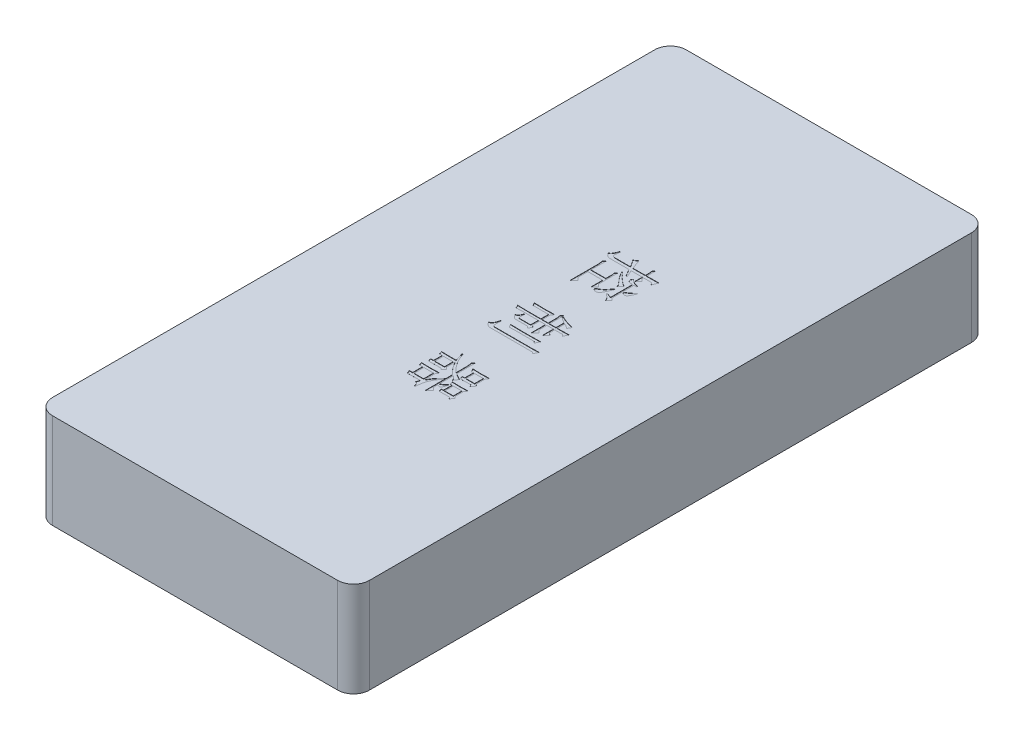
from build123d import *

# Parameters (mm, degrees)
SKETCH_1_W          = 100
SKETCH_1_H          = 200
EXTRUDE_1_DEPTH     = 30
SKETCH_2_W          = 2.707191781
SKETCH_2_H          = 2.773972602
SKETCH_2_W_2        = 3.035958905
SKETCH_2_H_2        = 2.704623287
SKETCH_2_H_3        = 3.120719178
SKETCH_2_H_4        = 2.704623288
CUT_EXTRUDE_1_DEPTH = 0.1
FILLET_1_R          = 5


with BuildPart() as part:
    # 草图1 → 凸台-拉伸1 (new body)
    with BuildSketch(Plane(origin=(0, 0, 0), x_dir=(1, 0, 0), z_dir=(0, 1, 0))):
        Rectangle(SKETCH_1_W, SKETCH_1_H)
    extrude(amount=EXTRUDE_1_DEPTH)

    # 草图2 → 切除-拉伸1 (cut)
    # profile 1 of 12: a face of its own
    with BuildSketch(Plane(origin=(0, 30, 0), x_dir=(1, 0, 0), z_dir=(0, 1, 0))):
        with BuildLine():
            Line((5.183219178, 28.225171233), (5.183219178, 22.122431507))
            Line((5.183219178, 22.122431507), (6.015410959, 21.290239726))
            Line((6.015410959, 21.290239726), (4.767123288, 20.041952055))
            Line((4.767123288, 20.041952055), (4.767123288, 23.856164384))
            Line((4.767123288, 23.856164384), (0.087328767, 23.856164384))
            Line((0.087328767, 23.856164384), (0.087328767, 20.735445205))
            Line((0.087328767, 20.735445205), (0.988869863, 19.83390411))
            Line((0.988869863, 19.83390411), (-0.328767123, 18.516267123))
            Line((-0.328767123, 18.516267123), (-0.328767123, 27.323630137))
            add(Edge.make_bspline(
                [(-0.328767123, 27.323630137), (-0.331222231, 27.470969524), (-0.336055453, 27.761027625), (-0.374434045, 28.186840132), (-0.441100052, 28.595216305), (-0.50519036, 28.858231521), (-0.536815068, 28.988013699)],
                knots=[0, 0, 0, 0, 1.051063684, 2.069165233, 3.04724927, 4, 4, 4, 4], degree=3))
            Line((-0.536815068, 28.988013699), (0.087328767, 29.612157534))
            Line((0.087328767, 29.612157534), (0.087328767, 24.827054795))
            Line((0.087328767, 24.827054795), (4.767123288, 24.827054795))
            Line((4.767123288, 24.827054795), (4.767123288, 26.907534247))
            Line((4.767123288, 26.907534247), (4.628424658, 27.670376712))
            Line((4.628424658, 27.670376712), (5.183219178, 28.225171233))
        make_face()
    # profile 2 of 12: a face of its own
    with BuildSketch(Plane(origin=(0, 30, 0), x_dir=(1, 0, 0), z_dir=(0, 1, 0))):
        with BuildLine():
            add(Edge.make_bspline(
                [(8.542808219, 25.03510274), (8.376646638, 25.212339659), (8.051168683, 25.559512031), (7.588261178, 26.084218642), (7.159350093, 26.599357915), (6.765167086, 27.106408408), (6.404887393, 27.604721332), (6.078806602, 28.094484294), (5.785963252, 28.575375992), (5.614083587, 28.898987622), (5.529965753, 29.057363014)],
                knots=[0, 0, 0, 0, 1.156336434, 2.26503634, 3.329987673, 4.346491992, 5.321449847, 6.25617807, 7.146574306, 8, 8, 8, 8], degree=3))
            Line((5.529965753, 29.057363014), (5.735445205, 29.196061644))
            add(Edge.make_bspline(
                [(5.735445205, 29.196061644), (5.894694178, 28.998561354), (6.208874123, 28.608915951), (6.702697463, 28.05789916), (7.203947953, 27.541875545), (7.715527871, 27.0654585), (8.231220495, 26.62054088), (8.759421691, 26.218268585), (9.293278031, 25.847271124), (9.662159734, 25.628837331), (9.845034247, 25.520547945)],
                knots=[0, 0, 0, 0, 1.097558762, 2.165357468, 3.200105271, 4.20915088, 5.189137413, 6.145661431, 7.080704579, 8, 8, 8, 8], degree=3))
            Line((9.845034247, 25.520547945), (8.748287671, 24.341609589))
            Line((8.748287671, 24.341609589), (8.542808219, 25.03510274))
        make_face()
    # profile 3 of 12: a face of its own
    with BuildSketch(Plane(origin=(0, 30, 0), x_dir=(1, 0, 0), z_dir=(0, 1, 0))):
        with BuildLine():
            Line((9.084760274, 23.440068493), (9.290239726, 23.301369863))
            add(Edge.make_bspline(
                [(9.290239726, 23.301369863), (9.223648725, 23.135201193), (9.095371311, 22.815102575), (8.907722276, 22.355604986), (8.722734215, 21.939626905), (8.555955778, 21.561709422), (8.39430184, 21.226592951), (8.238553221, 20.93459989), (8.100614274, 20.678927628), (7.964085458, 20.464821958), (7.834274765, 20.28179352), (7.706075626, 20.123421633), (7.575097714, 19.989507359), (7.442796139, 19.877557832), (7.310575683, 19.78617224), (7.173981441, 19.721399864), (7.037797088, 19.675937555), (6.860470802, 19.651676286), (6.653531877, 19.652804124), (6.428359558, 19.686376325), (6.234256199, 19.754831603), (6.082488329, 19.858623742), (5.969290469, 19.967974685), (5.885894603, 20.057455104), (5.826706918, 20.122116303), (5.812593293, 20.164823934), (5.807363014, 20.180650685)],
                knots=[0, 0, 0, 0, 2.221672789, 4.279714018, 6.159065882, 7.871185812, 9.406123815, 10.774929285, 11.978261759, 13.009953149, 13.923973529, 14.762023894, 15.535920093, 16.24471408, 16.910724515, 17.523775955, 18.115175145, 18.68469364, 19.736595478, 20.672886263, 21.499884634, 22.266083828, 22.935138511, 23.446257124, 23.79479193, 24, 24, 24, 24], degree=3))
            add(Edge.make_bspline(
                [(5.807363014, 20.180650685), (5.810118249, 20.205090596), (5.816036222, 20.257585101), (5.861037478, 20.33420556), (5.924887069, 20.416004902), (6.016860709, 20.500495884), (6.133717919, 20.586441882), (6.273602167, 20.680228979), (6.440702481, 20.776644891), (6.562255323, 20.840358044), (6.626712329, 20.874143836)],
                knots=[0, 0, 0, 0, 0.527456402, 1.132924005, 1.885971963, 2.778031796, 3.823941379, 5.027470183, 6.423727738, 8, 8, 8, 8], degree=3))
            add(Edge.make_bspline(
                [(6.626712329, 20.874143836), (6.715077877, 20.926506522), (6.901916206, 21.037221129), (7.177340855, 21.247209482), (7.465784246, 21.50108223), (7.765852947, 21.80123962), (8.080727959, 22.143849701), (8.404447389, 22.535147087), (8.744833364, 22.969386523), (8.968548113, 23.279154581), (9.084760274, 23.440068493)],
                knots=[0, 0, 0, 0, 0.688371872, 1.455479582, 2.318090961, 3.264097909, 4.300380693, 5.437681015, 6.668962925, 8, 8, 8, 8], degree=3))
        make_face()
    # profile 4 of 12: a face of its own
    with BuildSketch(Plane(origin=(0, 30, 0), x_dir=(1, 0, 0), z_dir=(0, 1, 0))):
        with BuildLine():
            Line((9.08989726, 21.012842466), (10.684931507, 20.38869863))
            Line((10.684931507, 20.38869863), (10.684931507, 27.392979452))
            add(Edge.make_bspline(
                [(10.684931507, 27.392979452), (10.585594464, 27.394008902), (10.397962234, 27.395953374), (10.130742246, 27.409148401), (9.893817521, 27.428022105), (9.686518773, 27.457597743), (9.505022111, 27.501130878), (9.358609934, 27.587500426), (9.235281189, 27.6971313), (9.157527176, 27.839811029), (9.098757349, 27.979072354), (9.059245675, 28.104652922), (9.025841878, 28.205500834), (9.02213676, 28.267803956), (9.020547945, 28.294520548)],
                knots=[0, 0, 0, 0, 1.658874866, 3.133356696, 4.468029939, 5.62470865, 6.634248992, 7.556475842, 8.436619168, 9.353732994, 10.238047638, 10.9615019, 11.554675115, 12, 12, 12, 12], degree=3))
            add(Edge.make_bspline(
                [(9.020547945, 28.294520548), (9.026851664, 28.347301506), (9.041298347, 28.468263391), (9.105556956, 28.612413685), (9.169935581, 28.725592039), (9.214056297, 28.791817714), (9.254567215, 28.83748963), (9.28546336, 28.845912345), (9.297945205, 28.849315068)],
                knots=[0, 0, 0, 0, 1.48119583, 3.394562111, 4.36050321, 5.118249749, 5.643778524, 6, 6, 6, 6], degree=3))
            add(Edge.make_bspline(
                [(9.297945205, 28.849315068), (9.338788264, 28.842646816), (9.437410889, 28.826545167), (9.593694866, 28.739200067), (9.783279812, 28.606575411), (9.916958518, 28.495246631), (9.991438356, 28.433219178)],
                knots=[0, 0, 0, 0, 0.602584801, 1.455045156, 2.582064183, 4, 4, 4, 4], degree=3))
            add(Edge.make_bspline(
                [(9.991438356, 28.433219178), (10.051505537, 28.387666347), (10.174083617, 28.294707456), (10.374801127, 28.172576313), (10.592293251, 28.061676287), (10.826700025, 27.961699777), (11.078948552, 27.87188316), (11.348445805, 27.793305748), (11.634274353, 27.722365136), (11.831940564, 27.687989713), (11.933219178, 27.670376712)],
                knots=[0, 0, 0, 0, 0.857780197, 1.750457547, 2.670233957, 3.635223603, 4.649507386, 5.716600804, 6.830050396, 8, 8, 8, 8], degree=3))
            Line((11.933219178, 27.670376712), (11.933219178, 27.392979452))
            Line((11.933219178, 27.392979452), (11.101027397, 27.392979452))
            Line((11.101027397, 27.392979452), (11.101027397, 20.38869863))
            Line((11.101027397, 20.38869863), (11.794520548, 19.83390411))
            Line((11.794520548, 19.83390411), (10.684931507, 18.724315068))
            add(Edge.make_bspline(
                [(10.684931507, 18.724315068), (10.678625125, 18.796858963), (10.665373408, 18.949296788), (10.57788829, 19.180819437), (10.438683459, 19.422110352), (10.246295966, 19.676593979), (9.998223404, 19.940881106), (9.699532723, 20.220357856), (9.346623951, 20.513121389), (9.087502997, 20.704253864), (8.95119863, 20.804794521)],
                knots=[0, 0, 0, 0, 0.62472621, 1.312748711, 2.108519513, 3.019978839, 4.05326984, 5.227074555, 6.541369034, 8, 8, 8, 8], degree=3))
            Line((8.95119863, 20.804794521), (9.08989726, 21.012842466))
        make_face()
    # profile 5 of 12: a face of its own
    with BuildSketch(Plane(origin=(0, 30, 0), x_dir=(1, 0, 0), z_dir=(0, 1, 0))):
        with BuildLine():
            Line((13.839041096, 25.72859589), (14.049657534, 25.58989726))
            add(Edge.make_bspline(
                [(14.049657534, 25.58989726), (13.998355409, 25.473429479), (13.899781006, 25.249642612), (13.757052598, 24.928531738), (13.620689185, 24.637472073), (13.491663455, 24.376187446), (13.375358464, 24.141846183), (13.263599397, 23.939182158), (13.165200735, 23.763698169), (13.070997207, 23.617019766), (12.981203706, 23.492550286), (12.885703675, 23.392190667), (12.786507326, 23.309475481), (12.680897429, 23.248562308), (12.572460664, 23.203235534), (12.458377658, 23.179317165), (12.340172783, 23.177650959), (12.184615468, 23.199529063), (12.008533838, 23.245436265), (11.828528924, 23.31177666), (11.685969826, 23.380018672), (11.567985585, 23.487206622), (11.478100418, 23.622137087), (11.456937871, 23.737053475), (11.447773973, 23.786815068)],
                knots=[0, 0, 0, 0, 1.969424768, 3.784148659, 5.437778933, 6.942807495, 8.293749131, 9.48542138, 10.524009878, 11.406038017, 12.182432982, 12.894681389, 13.544422139, 14.173853452, 14.774165472, 15.356216713, 15.965813955, 16.593569761, 17.782513801, 18.771850109, 19.566015896, 20.204171455, 21.222362531, 22, 22, 22, 22], degree=3))
            add(Edge.make_bspline(
                [(11.447773973, 23.786815068), (11.454969291, 23.823494246), (11.471228566, 23.906378259), (11.58239147, 24.009328448), (11.736755799, 24.114199254), (11.86751133, 24.171012747), (11.940924658, 24.202910959)],
                knots=[0, 0, 0, 0, 0.651610588, 1.472445797, 2.580892413, 4, 4, 4, 4], degree=3))
            add(Edge.make_bspline(
                [(11.940924658, 24.202910959), (12.002113249, 24.235599289), (12.132880854, 24.305458304), (12.331844204, 24.431688389), (12.545404115, 24.584426061), (12.773847927, 24.763195051), (13.021095401, 24.964417534), (13.278359846, 25.198431868), (13.557827823, 25.45045105), (13.743032544, 25.633634927), (13.839041096, 25.72859589)],
                knots=[0, 0, 0, 0, 0.681165141, 1.455734343, 2.312029879, 3.258982338, 4.304417023, 5.441970212, 6.673939121, 8, 8, 8, 8], degree=3))
        make_face()
    # profile 6 of 12: a face of its own
    with BuildSketch(Plane(origin=(0, 30, 0), x_dir=(1, 0, 0), z_dir=(0, 1, 0))):
        with BuildLine():
            Line((7.348458904, 28.641267123), (5.961472603, 30.929794521))
            Line((5.961472603, 30.929794521), (-0.074486301, 30.929794521))
            add(Edge.make_bspline(
                [(-0.074486301, 30.929794521), (-0.164824307, 30.939134956), (-0.342902821, 30.957547262), (-0.600701476, 31.030972586), (-0.841997975, 31.143850647), (-1.069559581, 31.290427908), (-1.279849745, 31.477073519), (-1.475030167, 31.698500275), (-1.652965086, 31.958466589), (-1.755218984, 32.148785498), (-1.808219178, 32.247431507)],
                knots=[0, 0, 0, 0, 0.951282364, 1.875212421, 2.79533767, 3.736905861, 4.704203426, 5.734873166, 6.825940502, 8, 8, 8, 8], degree=3))
            add(Edge.make_bspline(
                [(-1.808219178, 32.247431507), (-1.743661316, 32.254408792), (-1.607988252, 32.269072068), (-1.414161718, 32.381867602), (-1.230169405, 32.556906638), (-1.047363731, 32.796639989), (-0.866570948, 33.101028654), (-0.692191425, 33.474410835), (-0.514363568, 33.911249201), (-0.408215019, 34.228761314), (-0.351883562, 34.397260274)],
                knots=[0, 0, 0, 0, 0.567410724, 1.192455101, 1.93008711, 2.801753461, 3.841774178, 5.047670883, 6.433242804, 8, 8, 8, 8], degree=3))
            Line((-0.351883562, 34.397260274), (-0.074486301, 34.397260274))
            add(Edge.make_bspline(
                [(-0.074486301, 34.397260274), (-0.096180139, 34.27573686), (-0.137687269, 34.043224372), (-0.192418077, 33.710367827), (-0.233136049, 33.409602669), (-0.26449175, 33.142473477), (-0.28571328, 32.907823907), (-0.296438781, 32.705606928), (-0.297823985, 32.534889084), (-0.287400086, 32.392945375), (-0.256978945, 32.271527999), (-0.196575629, 32.167074712), (-0.101159367, 32.085328082), (0.015912536, 32.013850342), (0.163718597, 31.965299938), (0.336460551, 31.926690807), (0.53797837, 31.904487528), (0.681456841, 31.90200449), (0.757705479, 31.900684932)],
                knots=[0, 0, 0, 0, 1.808220358, 3.459693913, 4.940655569, 6.253580308, 7.399219139, 8.391232753, 9.218943302, 9.899057853, 10.471018597, 11.038839643, 11.633582565, 12.291719892, 13.037465463, 13.898517392, 14.883210947, 16, 16, 16, 16], degree=3))
            Line((0.757705479, 31.900684932), (5.476027397, 31.900684932))
            add(Edge.make_bspline(
                [(5.476027397, 31.900684932), (5.387279249, 32.053253171), (5.219165187, 32.342260515), (4.977092399, 32.748147274), (4.753648866, 33.098620762), (4.550909315, 33.39363921), (4.372753949, 33.637698587), (4.213368595, 33.824524706), (4.080629672, 33.965673606), (3.987328723, 34.025254498), (3.947773973, 34.050513699)],
                knots=[0, 0, 0, 0, 1.596009153, 3.023292197, 4.273176395, 5.353314463, 6.260656545, 7.002131711, 7.576955733, 8, 8, 8, 8], degree=3))
            Line((3.947773973, 34.050513699), (5.198630137, 34.882705479))
            add(Edge.make_bspline(
                [(5.198630137, 34.882705479), (5.218536503, 34.80632392), (5.262211434, 34.638741383), (5.348678885, 34.369342185), (5.457284305, 34.05905312), (5.585780257, 33.707148706), (5.735788222, 33.313688237), (5.903858187, 32.877824841), (6.097505211, 32.402148716), (6.235966683, 32.072633712), (6.308219178, 31.900684932)],
                knots=[0, 0, 0, 0, 0.594885919, 1.30519058, 2.131778393, 3.072962133, 4.12892683, 5.305816866, 6.59411104, 8, 8, 8, 8], degree=3))
            Line((6.308219178, 31.900684932), (10.191780822, 31.900684932))
            Line((10.191780822, 31.900684932), (10.191780822, 33.357020548))
            Line((10.191780822, 33.357020548), (10.053082192, 34.189212329))
            Line((10.053082192, 34.189212329), (10.607876712, 34.744006849))
            Line((10.607876712, 34.744006849), (10.607876712, 31.900684932))
            add(Edge.make_bspline(
                [(10.607876712, 31.900684932), (10.812502299, 31.900173097), (11.208918508, 31.899181533), (11.784245699, 31.906106579), (12.321934935, 31.910198029), (12.822812516, 31.917633807), (13.286807345, 31.929095444), (13.713304914, 31.937127371), (14.101909448, 31.954089387), (14.348460194, 31.964894065), (14.465753425, 31.970034247)],
                knots=[0, 0, 0, 0, 1.272643643, 2.465461797, 3.57841033, 4.61688262, 5.580919197, 6.465104001, 7.269793692, 8, 8, 8, 8], degree=3))
            Line((14.465753425, 31.970034247), (13.695205479, 30.23630137))
            Line((13.695205479, 30.23630137), (13.132705479, 30.929794521))
            Line((13.132705479, 30.929794521), (10.607876712, 30.929794521))
            Line((10.607876712, 30.929794521), (10.607876712, 30.375))
            Line((10.607876712, 30.375), (11.301369863, 29.681506849))
            Line((11.301369863, 29.681506849), (10.191780822, 28.571917808))
            Line((10.191780822, 28.571917808), (10.191780822, 30.929794521))
            Line((10.191780822, 30.929794521), (6.654965753, 30.929794521))
            Line((6.654965753, 30.929794521), (7.625856164, 28.779965753))
            Line((7.625856164, 28.779965753), (7.348458904, 28.641267123))
        make_face()
    # profile 7 of 12: a face of its own
    with BuildSketch(Plane(origin=(0, 30, 0), x_dir=(1, 0, 0), z_dir=(0, 1, 0))):
        with BuildLine():
            add(Edge.make_bspline(
                [(2.283390411, -2.773972603), (2.413525277, -2.779138257), (2.690037966, -2.790114323), (3.129174262, -2.806927272), (3.618156185, -2.814981024), (4.155788106, -2.826407606), (4.74227974, -2.833850207), (5.377569049, -2.837871333), (6.061631745, -2.845041755), (6.781678205, -2.842441289), (7.509429424, -2.845028482), (8.220032852, -2.837750537), (8.89898585, -2.833786562), (9.546260445, -2.826257586), (10.161806798, -2.814727931), (10.74580028, -2.806672891), (11.298808153, -2.789540892), (11.65667745, -2.779061837), (11.830479452, -2.773972603)],
                knots=[0, 0, 0, 0, 0.654692731, 1.391101799, 2.209012074, 3.112981841, 4.094341678, 5.15742433, 6.306581118, 7.533174739, 8.776983709, 9.964873981, 11.105423337, 12.19006718, 13.218828337, 14.200254234, 15.125939497, 16, 16, 16, 16], degree=3))
            Line((11.830479452, -2.773972603), (11.134417808, -4.230308219))
            Line((11.134417808, -4.230308219), (10.715753425, -3.675513699))
            Line((10.715753425, -3.675513699), (4.304794521, -3.675513699))
            add(Edge.make_bspline(
                [(4.304794521, -3.675513699), (4.213174442, -3.676839541), (4.010177401, -3.679777129), (3.674561834, -3.694055075), (3.278027432, -3.713681848), (2.993115252, -3.733998386), (2.840753425, -3.744863014)],
                knots=[0, 0, 0, 0, 0.750054126, 1.661849349, 2.749632581, 4, 4, 4, 4], degree=3))
            Line((2.840753425, -3.744863014), (2.283390411, -2.773972603))
        make_face()
    # profile 8 of 12: a face of its own
    with BuildSketch(Plane(origin=(0, 30, 0), x_dir=(1, 0, 0), z_dir=(0, 1, 0))):
        with BuildLine():
            add(Edge.make_bspline(
                [(12.310787671, -5.964041096), (12.675609545, -5.961004277), (13.394486909, -5.955020258), (14.112247807, -5.914599484), (14.465753425, -5.894691781)],
                knots=[0, 0, 0, 0, 1.014976663, 2, 2, 2, 2], degree=3))
            Line((14.465753425, -5.894691781), (13.769691781, -7.351027397))
            Line((13.769691781, -7.351027397), (13.284246575, -6.865582192))
            Line((13.284246575, -6.865582192), (0.27739726, -6.865582192))
            add(Edge.make_bspline(
                [(0.27739726, -6.865582192), (0.159909454, -6.867425772), (-0.067820902, -6.870999241), (-0.396779332, -6.817755838), (-0.701399164, -6.723220081), (-0.97820765, -6.577682341), (-1.228048986, -6.385822386), (-1.454808255, -6.152363256), (-1.650343414, -5.868831569), (-1.75441376, -5.657306038), (-1.808219178, -5.547945205)],
                knots=[0, 0, 0, 0, 1.065221631, 2.064752996, 3.011361688, 3.950276852, 4.887903625, 5.861084974, 6.894159364, 8, 8, 8, 8], degree=3))
            add(Edge.make_bspline(
                [(-1.808219178, -5.547945205), (-1.71769589, -5.530231588), (-1.537265826, -5.494924993), (-1.288150534, -5.357949922), (-1.067464365, -5.159500438), (-0.871355512, -4.900036246), (-0.702745802, -4.578147708), (-0.558282753, -4.194761603), (-0.435809545, -3.749154079), (-0.377521644, -3.428642657), (-0.346746575, -3.259417808)],
                knots=[0, 0, 0, 0, 0.758687152, 1.512207249, 2.314469735, 3.197766889, 4.185671758, 5.308103181, 6.578722005, 8, 8, 8, 8], degree=3))
            Line((-0.346746575, -3.259417808), (-0.069349315, -3.259417808))
            add(Edge.make_bspline(
                [(-0.069349315, -3.259417808), (-0.08014622, -3.465731971), (-0.100391104, -3.852584155), (-0.121014891, -4.394570135), (-0.132584915, -4.858796221), (-0.142246698, -5.19585442), (-0.134355382, -5.427447005), (-0.099872076, -5.570497533), (-0.048395624, -5.694921952), (0.033662936, -5.792752525), (0.132159842, -5.872283412), (0.255320599, -5.925916498), (0.398835334, -5.959959827), (0.502344179, -5.962624645), (0.557363014, -5.964041096)],
                knots=[0, 0, 0, 0, 2.369720351, 4.443376459, 6.221600866, 7.694836481, 8.314786265, 8.869807763, 9.375359127, 9.84315846, 10.318626306, 10.815227448, 11.370248947, 12, 12, 12, 12], degree=3))
            Line((0.557363014, -5.964041096), (12.310787671, -5.964041096))
        make_face()
    # profile 9 of 12: a face of its own
    with BuildSketch(Plane(origin=(0, 30, 0), x_dir=(1, 0, 0), z_dir=(0, 1, 0))):
        with BuildLine():
            Line((10.772260274, 3.536815068), (11.817636986, 3.536815068))
            add(Edge.make_bspline(
                [(11.817636986, 3.536815068), (11.952914357, 3.536309005), (12.215774918, 3.535325661), (12.597601713, 3.542224887), (12.956359998, 3.546383213), (13.290300135, 3.553670441), (13.601012397, 3.565336455), (13.887164276, 3.573250327), (14.149863841, 3.590271477), (14.316782287, 3.601031664), (14.39640411, 3.606164384)],
                knots=[0, 0, 0, 0, 1.258249954, 2.444934331, 3.551990324, 4.595496403, 5.551660039, 6.444152705, 7.257844778, 8, 8, 8, 8], degree=3))
            Line((14.39640411, 3.606164384), (13.769691781, 2.149828767))
            Line((13.769691781, 2.149828767), (13.281678082, 2.704623288))
            Line((13.281678082, 2.704623288), (10.772260274, 2.704623288))
            Line((10.772260274, 2.704623288), (10.772260274, 1.109589041))
            Line((10.772260274, 1.109589041), (11.604452055, 0.346746575))
            Line((11.604452055, 0.346746575), (10.356164384, -0.901541096))
            Line((10.356164384, -0.901541096), (10.356164384, 2.704623288))
            Line((10.356164384, 2.704623288), (8.306506849, 2.704623288))
            Line((8.306506849, 2.704623288), (8.306506849, 0.208047945))
            Line((8.306506849, 0.208047945), (9.13869863, -0.624143836))
            Line((9.13869863, -0.624143836), (7.890410959, -1.872431507))
            Line((7.890410959, -1.872431507), (7.890410959, 2.704623288))
            Line((7.890410959, 2.704623288), (6.005136986, 2.704623288))
            Line((6.005136986, 2.704623288), (6.005136986, 0.41609589))
            Line((6.005136986, 0.41609589), (6.698630137, -0.069349315))
            Line((6.698630137, -0.069349315), (5.935787671, -1.109589041))
            Line((5.935787671, -1.109589041), (5.450342466, -0.554794521))
            Line((5.450342466, -0.554794521), (2.052226027, -0.554794521))
            add(Edge.make_bspline(
                [(2.052226027, -0.554794521), (1.951799918, -0.556758138), (1.75795417, -0.560548376), (1.477586827, -0.505799146), (1.218672963, -0.412554331), (0.987030145, -0.264725874), (0.781766381, -0.072264486), (0.596752769, 0.161832933), (0.440978323, 0.445068168), (0.360492448, 0.653879913), (0.318493151, 0.762842466)],
                knots=[0, 0, 0, 0, 1.017401403, 1.963821335, 2.88272422, 3.796967302, 4.73217852, 5.728861945, 6.814870297, 8, 8, 8, 8], degree=3))
            add(Edge.make_bspline(
                [(0.318493151, 0.762842466), (0.381195868, 0.756244018), (0.505097337, 0.743205391), (0.691155537, 0.795516534), (0.865470931, 0.899799876), (1.02392374, 1.063339764), (1.176685619, 1.275241857), (1.31775392, 1.541435532), (1.45177456, 1.860597348), (1.526743765, 2.094345598), (1.566780822, 2.219178082)],
                knots=[0, 0, 0, 0, 0.719770975, 1.422277761, 2.177514121, 3.034373414, 4.021596162, 5.176584016, 6.492163977, 8, 8, 8, 8], degree=3))
            Line((1.566780822, 2.219178082), (1.844178082, 2.219178082))
            add(Edge.make_bspline(
                [(1.844178082, 2.219178082), (1.822457572, 2.058349695), (1.782308879, 1.761070783), (1.743623071, 1.35039641), (1.712723694, 1.014081944), (1.701465034, 0.779330619), (1.710276097, 0.623098045), (1.744918094, 0.52855975), (1.800349085, 0.447277747), (1.88098411, 0.386370122), (1.979634393, 0.335647079), (2.100822925, 0.301430149), (2.243362368, 0.281813348), (2.344963854, 0.278929983), (2.398972603, 0.27739726)],
                knots=[0, 0, 0, 0, 2.400018075, 4.436248949, 6.100977197, 7.393190724, 7.914850402, 8.399541632, 8.863266875, 9.349774361, 9.876481736, 10.497499308, 11.201309097, 12, 12, 12, 12], degree=3))
            Line((2.398972603, 0.27739726), (5.589041096, 0.27739726))
            Line((5.589041096, 0.27739726), (5.589041096, 2.704623288))
            Line((5.589041096, 2.704623288), (0.773116438, 2.704623288))
            add(Edge.make_bspline(
                [(0.773116438, 2.704623288), (0.581325809, 2.70353963), (0.208831744, 2.701434959), (-0.332306349, 2.688038259), (-0.838556602, 2.669538697), (-1.163575829, 2.646416679), (-1.320205479, 2.635273973)],
                knots=[0, 0, 0, 0, 1.098589798, 2.133671401, 3.100599682, 4, 4, 4, 4], degree=3))
            Line((-1.320205479, 2.635273973), (-1.808219178, 3.606164384))
            add(Edge.make_bspline(
                [(-1.808219178, 3.606164384), (-1.618999138, 3.601309102), (-1.258525304, 3.592059543), (-0.744074185, 3.57447769), (-0.281652014, 3.566122658), (0.128406952, 3.554967497), (0.486281039, 3.546777537), (0.791113806, 3.543147054), (1.043635119, 3.535704526), (1.194345694, 3.536474063), (1.261130137, 3.536815068)],
                knots=[0, 0, 0, 0, 1.479627748, 2.818766372, 4.023746565, 5.094910282, 6.025409737, 6.82195138, 7.477970797, 8, 8, 8, 8], degree=3))
            Line((1.261130137, 3.536815068), (5.589041096, 3.536815068))
            Line((5.589041096, 3.536815068), (5.589041096, 5.964041096))
            Line((5.589041096, 5.964041096), (0.665239726, 5.964041096))
            Line((0.665239726, 5.964041096), (0.179794521, 6.865582192))
            add(Edge.make_bspline(
                [(0.179794521, 6.865582192), (0.476004874, 6.854581036), (1.059773217, 6.83290007), (1.922027017, 6.813400284), (2.758518175, 6.800353291), (3.568492538, 6.79424909), (4.353646076, 6.800050311), (5.112236402, 6.812886359), (5.845264166, 6.831922592), (6.324517252, 6.854494586), (6.559931507, 6.865582192)],
                knots=[0, 0, 0, 0, 1.114655832, 2.196752345, 3.243250355, 4.260668401, 5.242671441, 6.195812807, 7.113763906, 8, 8, 8, 8], degree=3))
            Line((6.559931507, 6.865582192), (6.005136986, 5.894691781))
            Line((6.005136986, 5.894691781), (6.005136986, 3.536815068))
            Line((6.005136986, 3.536815068), (7.890410959, 3.536815068))
            Line((7.890410959, 3.536815068), (7.890410959, 5.825342466))
            add(Edge.make_bspline(
                [(7.890410959, 5.825342466), (7.887955851, 5.972681852), (7.88312263, 6.262739953), (7.844744038, 6.688552461), (7.77807803, 7.096928633), (7.713987723, 7.35994385), (7.682363014, 7.489726027)],
                knots=[0, 0, 0, 0, 1.051063684, 2.069165233, 3.04724927, 4, 4, 4, 4], degree=3))
            Line((7.682363014, 7.489726027), (8.306506849, 8.113869863))
            Line((8.306506849, 8.113869863), (8.306506849, 3.536815068))
            Line((8.306506849, 3.536815068), (10.356164384, 3.536815068))
            Line((10.356164384, 3.536815068), (10.356164384, 6.033390411))
            add(Edge.make_bspline(
                [(10.356164384, 6.033390411), (10.167551486, 6.147226366), (9.802639568, 6.367466324), (9.291482872, 6.715353111), (8.82870525, 7.059745018), (8.549127298, 7.303093781), (8.414383562, 7.420376712)],
                knots=[0, 0, 0, 0, 1.105905581, 2.139610442, 3.10337765, 4, 4, 4, 4], degree=3))
            Line((8.414383562, 7.420376712), (8.483732877, 7.628424658))
            add(Edge.make_bspline(
                [(8.483732877, 7.628424658), (8.718404222, 7.517968735), (9.170060807, 7.305381448), (9.83499238, 7.025919401), (10.45449517, 6.785820427), (11.032294389, 6.589487319), (11.565534908, 6.432469624), (12.05572945, 6.311148503), (12.501784286, 6.219611722), (12.787384084, 6.187319753), (12.922089041, 6.172089041)],
                knots=[0, 0, 0, 0, 1.326489263, 2.553007103, 3.688326024, 4.724181207, 5.673409887, 6.530529915, 7.306915108, 8, 8, 8, 8], degree=3))
            Line((12.922089041, 6.172089041), (12.22859589, 4.854452055))
            add(Edge.make_bspline(
                [(12.22859589, 4.854452055), (12.20692405, 4.896485649), (12.160914747, 4.985722943), (12.054933151, 5.109517348), (11.922028871, 5.237233078), (11.754923803, 5.365721423), (11.556175149, 5.496101968), (11.324957895, 5.629697512), (11.059200112, 5.761549019), (10.87092668, 5.848909648), (10.772260274, 5.894691781)],
                knots=[0, 0, 0, 0, 0.621409584, 1.319252158, 2.133225883, 3.049619521, 4.091735985, 5.264563186, 6.566469424, 8, 8, 8, 8], degree=3))
            Line((10.772260274, 5.894691781), (10.772260274, 3.536815068))
        make_face()
    # profile 10 of 12: a face of its own
    with BuildSketch(Plane(origin=(0, 30, 0), x_dir=(1, 0, 0), z_dir=(0, 1, 0))):
        with BuildLine():
            add(Edge.make_bspline(
                [(8.519691781, -20.874143836), (8.976814017, -20.893572424), (9.883079224, -20.932090465), (11.226871885, -20.948882904), (12.533089969, -20.933413629), (13.388775455, -20.893640168), (13.808219178, -20.874143836)],
                knots=[0, 0, 0, 0, 1.037682106, 2.057251022, 3.047694652, 4, 4, 4, 4], degree=3))
            Line((13.808219178, -20.874143836), (13.238013699, -21.845034247))
            Line((13.238013699, -21.845034247), (13.238013699, -24.549657534))
            Line((13.238013699, -24.549657534), (13.808219178, -25.03510274))
            Line((13.808219178, -25.03510274), (12.916952055, -26.144691781))
            Line((12.916952055, -26.144691781), (12.505993151, -25.520547945))
            add(Edge.make_bspline(
                [(12.505993151, -25.520547945), (12.309072808, -25.520012059), (11.934059748, -25.518991524), (11.398116023, -25.5258661), (10.9152206, -25.529991044), (10.485389284, -25.537125754), (10.108737124, -25.548714498), (9.785776719, -25.556533118), (9.516149019, -25.572751559), (9.354440996, -25.584619804), (9.282534247, -25.58989726)],
                knots=[0, 0, 0, 0, 1.465492511, 2.790868742, 3.98881736, 5.05943472, 5.990052949, 6.793292427, 7.46341302, 8, 8, 8, 8], degree=3))
            Line((9.282534247, -25.58989726), (8.866438356, -24.619006849))
            Line((8.866438356, -24.619006849), (9.698630137, -24.619006849))
            Line((9.698630137, -24.619006849), (9.698630137, -21.845034247))
            Line((9.698630137, -21.845034247), (9.005136986, -21.845034247))
            Line((9.005136986, -21.845034247), (8.519691781, -20.874143836))
        make_face()
        with Locations((11.468321918, -23.232020548)):
            Rectangle(SKETCH_2_W, SKETCH_2_H, mode=Mode.SUBTRACT)
    # profile 11 of 12: a face of its own
    with BuildSketch(Plane(origin=(0, 30, 0), x_dir=(1, 0, 0), z_dir=(0, 1, 0))):
        with BuildLine():
            add(Edge.make_bspline(
                [(3.274828767, -32.316780822), (3.044518416, -32.316252763), (2.603582717, -32.315241779), (1.971746505, -32.322114096), (1.398099896, -32.32622207), (0.881806332, -32.333508177), (0.422948626, -32.34495996), (0.021264206, -32.352938282), (-0.321992014, -32.369314548), (-0.531684865, -32.380886172), (-0.626712329, -32.386130137)],
                knots=[0, 0, 0, 0, 1.416318962, 2.711582825, 3.885753199, 4.944161445, 5.886854328, 6.708483985, 7.414717805, 8, 8, 8, 8], degree=3))
            Line((-0.626712329, -32.386130137), (-1.037671233, -31.345890411))
            Line((-1.037671233, -31.345890411), (0, -31.345890411))
            Line((0, -31.345890411), (0, -28.225171233))
            Line((0, -28.225171233), (-0.98630137, -28.225171233))
            Line((-0.98630137, -28.225171233), (-1.315068493, -27.254280822))
            add(Edge.make_bspline(
                [(-1.315068493, -27.254280822), (-0.827119992, -27.273714464), (0.141670025, -27.312298698), (1.580469345, -27.329011626), (2.982536784, -27.313529486), (3.902468655, -27.273775741), (4.35359589, -27.254280822)],
                knots=[0, 0, 0, 0, 1.033329117, 2.051607763, 3.044524022, 4, 4, 4, 4], degree=3))
            Line((4.35359589, -27.254280822), (3.868150685, -28.225171233))
            Line((3.868150685, -28.225171233), (3.868150685, -31.137842466))
            Line((3.868150685, -31.137842466), (3.999143836, -31.276541096))
            add(Edge.make_bspline(
                [(3.999143836, -31.276541096), (4.10450638, -31.085515396), (4.311088689, -30.710974987), (4.643325785, -30.175899433), (4.986445526, -29.676736303), (5.344474252, -29.215715723), (5.714366777, -28.790601875), (6.096944977, -28.402941539), (6.490091597, -28.049854379), (6.767266114, -27.842231334), (6.904109589, -27.739726027)],
                knots=[0, 0, 0, 0, 1.133958455, 2.223330485, 3.272754102, 4.281462526, 5.25620255, 6.200395149, 7.111519401, 8, 8, 8, 8], degree=3))
            Line((6.904109589, -27.739726027), (6.904109589, -25.659246575))
            add(Edge.make_bspline(
                [(6.904109589, -25.659246575), (6.737510349, -25.508293835), (6.408934128, -25.210576505), (5.945264947, -24.744145838), (5.515234784, -24.266219759), (5.120478055, -23.775626062), (4.756259879, -23.275512614), (4.424653006, -22.765392783), (4.127727575, -22.242591207), (3.95441501, -21.884547654), (3.868150685, -21.706335616)],
                knots=[0, 0, 0, 0, 1.074575135, 2.119336413, 3.142419922, 4.146597735, 5.128167811, 6.098797509, 7.053698452, 8, 8, 8, 8], degree=3))
            Line((3.868150685, -21.706335616), (3.868150685, -24.619006849))
            Line((3.868150685, -24.619006849), (4.492294521, -25.104452055))
            Line((4.492294521, -25.104452055), (3.657534247, -26.144691781))
            Line((3.657534247, -26.144691781), (3.23630137, -25.659246575))
            add(Edge.make_bspline(
                [(3.23630137, -25.659246575), (3.001710241, -25.658717876), (2.553069261, -25.657706772), (1.912670815, -25.664544339), (1.335599873, -25.668668986), (0.821873007, -25.675914824), (0.371576623, -25.687320215), (-0.015561044, -25.695298286), (-0.33828243, -25.711463251), (-0.532543386, -25.723319017), (-0.619006849, -25.72859589)],
                knots=[0, 0, 0, 0, 1.459913289, 2.791993585, 3.985546911, 5.051296926, 5.989293604, 6.788800325, 7.460908045, 8, 8, 8, 8], degree=3))
            Line((-0.619006849, -25.72859589), (-0.968321918, -24.757705479))
            Line((-0.968321918, -24.757705479), (0, -24.757705479))
            Line((0, -24.757705479), (0, -22.053082192))
            Line((0, -22.053082192), (-0.850171233, -22.053082192))
            Line((-0.850171233, -22.053082192), (-1.176369863, -21.082191781))
            add(Edge.make_bspline(
                [(-1.176369863, -21.082191781), (-0.979488597, -21.093271055), (-0.580748551, -21.115709707), (0.026446229, -21.134767441), (0.650623942, -21.147962165), (1.281672095, -21.152488665), (1.895547738, -21.151313094), (2.470034295, -21.151594221), (2.99229451, -21.151529839), (3.323630134, -21.151537482), (3.480308219, -21.151541096)],
                knots=[0, 0, 0, 0, 1.015988255, 2.057662525, 3.129845098, 4.232715445, 5.309082461, 6.292811332, 7.192724738, 8, 8, 8, 8], degree=3))
            add(Edge.make_bspline(
                [(3.480308219, -21.151541096), (3.403921852, -20.923283878), (3.253700804, -20.474394373), (3.050147592, -19.807003974), (2.874489148, -19.156797638), (2.776067644, -18.727208371), (2.727739726, -18.516267123)],
                knots=[0, 0, 0, 0, 1.053319498, 2.071452874, 3.053025371, 4, 4, 4, 4], degree=3))
            Line((2.727739726, -18.516267123), (2.933219178, -18.446917808))
            add(Edge.make_bspline(
                [(2.933219178, -18.446917808), (3.048799426, -18.761630622), (3.275018102, -19.377600197), (3.664626431, -20.258299328), (4.079676283, -21.080238785), (4.529566524, -21.848273393), (5.032399525, -22.570101575), (5.590298523, -23.263278666), (6.215861268, -23.927622676), (6.672578039, -24.340400656), (6.904109589, -24.549657534)],
                knots=[0, 0, 0, 0, 1.091529556, 2.136389009, 3.13388342, 4.088761362, 5.032305721, 5.995890833, 6.984021318, 8, 8, 8, 8], degree=3))
            Line((6.904109589, -24.549657534), (6.904109589, -21.220890411))
            add(Edge.make_bspline(
                [(6.904109589, -21.220890411), (6.901654481, -21.073551024), (6.89682126, -20.783492923), (6.858442668, -20.357680416), (6.79177666, -19.949304243), (6.727686353, -19.686289026), (6.696061644, -19.556506849)],
                knots=[0, 0, 0, 0, 1.051063684, 2.069165233, 3.04724927, 4, 4, 4, 4], degree=3))
            Line((6.696061644, -19.556506849), (7.320205479, -18.932363014))
            Line((7.320205479, -18.932363014), (7.320205479, -24.757705479))
            add(Edge.make_bspline(
                [(7.320205479, -24.757705479), (7.482987394, -24.85997629), (7.807826205, -25.064062404), (8.307865868, -25.347582251), (8.813261647, -25.619885712), (9.158545729, -25.784777848), (9.331335616, -25.867294521)],
                knots=[0, 0, 0, 0, 1.003539972, 2.002610255, 3.000449866, 4, 4, 4, 4], degree=3))
            Line((9.331335616, -25.867294521), (8.429794521, -27.184931507))
            add(Edge.make_bspline(
                [(8.429794521, -27.184931507), (8.376355228, -27.068774416), (8.265138417, -26.827030546), (8.011136017, -26.495007844), (7.699768675, -26.164016978), (7.450734069, -25.969334877), (7.320205479, -25.867294521)],
                knots=[0, 0, 0, 0, 0.877877114, 1.827020706, 2.861058199, 4, 4, 4, 4], degree=3))
            Line((7.320205479, -25.867294521), (7.320205479, -30.23630137))
            add(Edge.make_bspline(
                [(7.320205479, -30.23630137), (7.400475177, -30.205242345), (7.560791578, -30.143210579), (7.791000657, -30.022984121), (8.012844547, -29.881290435), (8.224664689, -29.716501796), (8.429936474, -29.532886304), (8.62496562, -29.326128705), (8.812853714, -29.098343604), (8.926707082, -28.933248059), (8.984589041, -28.849315068)],
                knots=[0, 0, 0, 0, 0.936454216, 1.870306908, 2.821855806, 3.798815043, 4.788893157, 5.81745103, 6.890413056, 8, 8, 8, 8], degree=3))
            Line((8.984589041, -28.849315068), (9.192636986, -28.988013699))
            add(Edge.make_bspline(
                [(9.192636986, -28.988013699), (9.165072896, -29.092662953), (9.112252792, -29.293198665), (9.025960578, -29.576530703), (8.949229288, -29.831542436), (8.86737941, -30.054098899), (8.792485313, -30.24770673), (8.718903487, -30.411747632), (8.643798002, -30.54286649), (8.555966724, -30.675412907), (8.446010372, -30.798454542), (8.319919874, -30.908178013), (8.201932357, -30.984677186), (8.119787599, -30.994673109), (8.083047945, -30.999143836)],
                knots=[0, 0, 0, 0, 1.623594058, 3.111236623, 4.443931417, 5.618313478, 6.667958308, 7.558915311, 8.312599909, 8.932567449, 9.942876071, 10.771947044, 11.45074717, 12, 12, 12, 12], degree=3))
            add(Edge.make_bspline(
                [(8.083047945, -30.999143836), (8.023387329, -30.995152427), (7.897169429, -30.986708209), (7.708873313, -30.912225954), (7.510959268, -30.804092249), (7.386424278, -30.705057078), (7.320205479, -30.65239726)],
                knots=[0, 0, 0, 0, 0.83591848, 1.768467722, 2.813430787, 4, 4, 4, 4], degree=3))
            Line((7.320205479, -30.65239726), (7.320205479, -32.039383562))
            Line((7.320205479, -32.039383562), (8.29109589, -33.010273973))
            Line((8.29109589, -33.010273973), (6.904109589, -34.397260274))
            Line((6.904109589, -34.397260274), (6.904109589, -28.155821918))
            add(Edge.make_bspline(
                [(6.904109589, -28.155821918), (6.725172142, -28.357640821), (6.365280929, -28.76355278), (5.883465593, -29.4294159), (5.440882453, -30.139614578), (5.108579002, -30.767748054), (4.871324904, -31.299450479), (4.71454908, -31.723938604), (4.581869996, -32.172217241), (4.468874981, -32.642931905), (4.377261997, -33.135977923), (4.304608506, -33.651743062), (4.256420127, -34.190167983), (4.240814456, -34.557278164), (4.232876712, -34.744006849)],
                knots=[0, 0, 0, 0, 1.33304205, 2.681105198, 4.057892879, 5.468693142, 6.190848033, 6.935594602, 7.704426823, 8.501248572, 9.328257948, 10.183228506, 11.075908627, 12, 12, 12, 12], degree=3))
            Line((4.232876712, -34.744006849), (3.960616438, -34.744006849))
            add(Edge.make_bspline(
                [(3.960616438, -34.744006849), (3.948308857, -34.655359721), (3.924843424, -34.486346555), (3.855698826, -34.250002349), (3.771214167, -34.039748125), (3.658068493, -33.85977447), (3.526762033, -33.705879249), (3.373422928, -33.580389359), (3.196767625, -33.485573588), (3.068467939, -33.446460028), (3.002568493, -33.426369863)],
                knots=[0, 0, 0, 0, 1.23066855, 2.346372543, 3.381972326, 4.340420049, 5.259791277, 6.156433905, 7.053076533, 8, 8, 8, 8], degree=3))
            Line((3.002568493, -33.426369863), (3.344178082, -32.386130137))
            Line((3.344178082, -32.386130137), (3.274828767, -32.316780822))
        make_face()
        with Locations((1.934075342, -23.405393835)):
            Rectangle(SKETCH_2_W_2, SKETCH_2_H_2, mode=Mode.SUBTRACT)
        with Locations((1.934075342, -29.785530822)):
            Rectangle(SKETCH_2_W_2, SKETCH_2_H_3, mode=Mode.SUBTRACT)
    # profile 12 of 12: a face of its own
    with BuildSketch(Plane(origin=(0, 30, 0), x_dir=(1, 0, 0), z_dir=(0, 1, 0))):
        with BuildLine():
            add(Edge.make_bspline(
                [(8.866438356, -27.670376712), (9.285883046, -27.689848988), (10.129597501, -27.72901754), (11.393828677, -27.744966453), (12.640135804, -27.729743413), (13.460696219, -27.689879994), (13.862157534, -27.670376712)],
                knots=[0, 0, 0, 0, 1.008067256, 2.027730795, 3.035062165, 4, 4, 4, 4], degree=3))
            Line((13.862157534, -27.670376712), (13.238013699, -28.641267123))
            Line((13.238013699, -28.641267123), (13.238013699, -31.276541096))
            Line((13.238013699, -31.276541096), (13.808219178, -31.761986301))
            Line((13.808219178, -31.761986301), (12.98630137, -32.802226027))
            Line((12.98630137, -32.802226027), (12.505993151, -32.247431507))
            add(Edge.make_bspline(
                [(12.505993151, -32.247431507), (12.324483631, -32.246907655), (11.976010818, -32.245901933), (11.475171331, -32.252782323), (11.017103021, -32.256903519), (10.601830839, -32.264173663), (10.22860314, -32.275724709), (9.897948982, -32.283623335), (9.610371169, -32.300197099), (9.433212702, -32.311563009), (9.351883562, -32.316780822)],
                knots=[0, 0, 0, 0, 1.380527048, 2.650418242, 3.809613174, 4.864725091, 5.809312706, 6.649754134, 7.380134987, 8, 8, 8, 8], degree=3))
            Line((9.351883562, -32.316780822), (9.005136986, -31.345890411))
            Line((9.005136986, -31.345890411), (9.698630137, -31.345890411))
            Line((9.698630137, -31.345890411), (9.698630137, -28.641267123))
            Line((9.698630137, -28.641267123), (9.213184932, -28.641267123))
            Line((9.213184932, -28.641267123), (8.866438356, -27.670376712))
        make_face()
        with Locations((11.468321918, -29.993578767)):
            Rectangle(SKETCH_2_W, SKETCH_2_H_4, mode=Mode.SUBTRACT)
    extrude(amount=-CUT_EXTRUDE_1_DEPTH, mode=Mode.SUBTRACT)

    # 圆角1
    fillet_1_edges = [part.edges().sort_by_distance(p)[0] for p in [
        (50, 15, 100),
        (-50, 15, 100),
        (-50, 15, -100),
        (50, 15, -100),
    ]]
    fillet(fillet_1_edges, radius=FILLET_1_R)


solid = part.part
